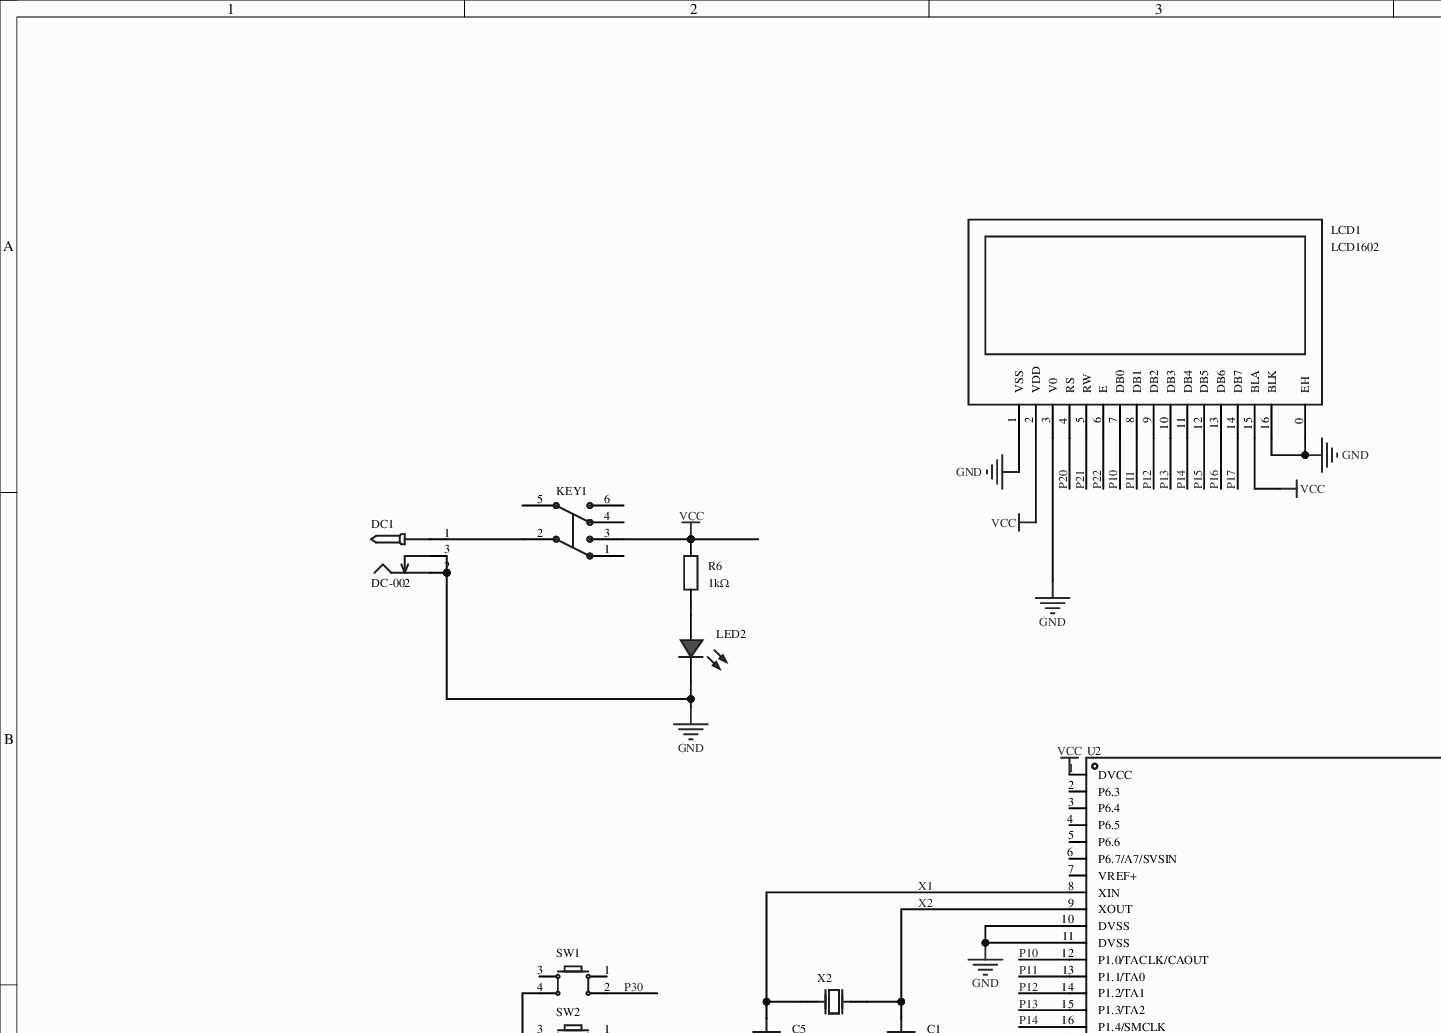
[diagram p0: MISC51174-3.schdoc, top left]
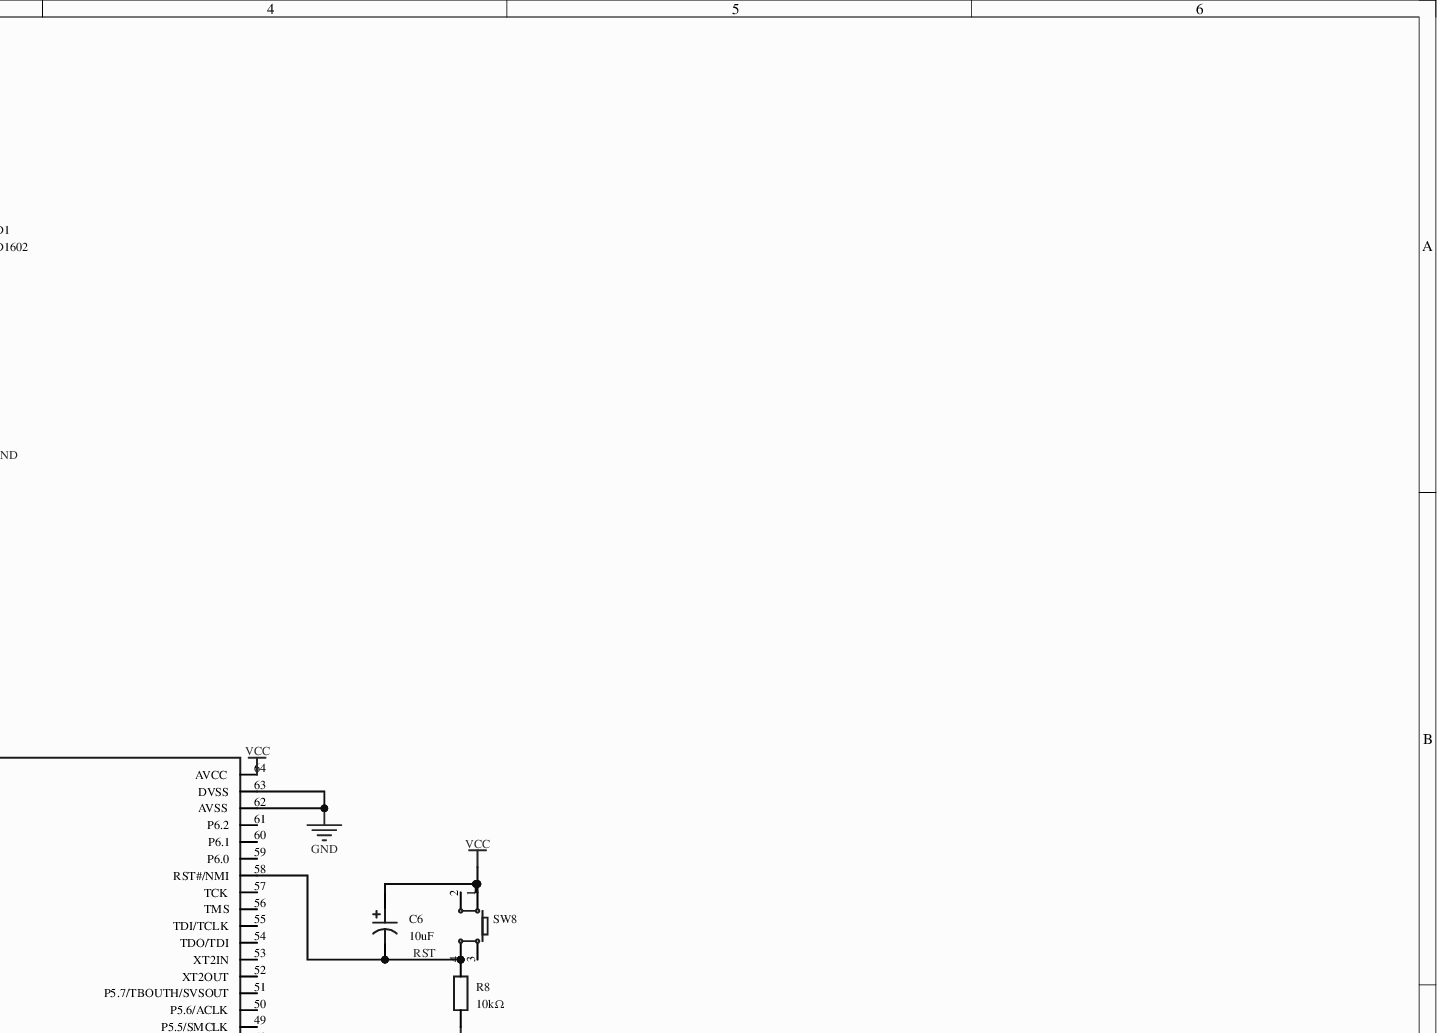
[diagram p1: MISC51174-3.schdoc, top right]
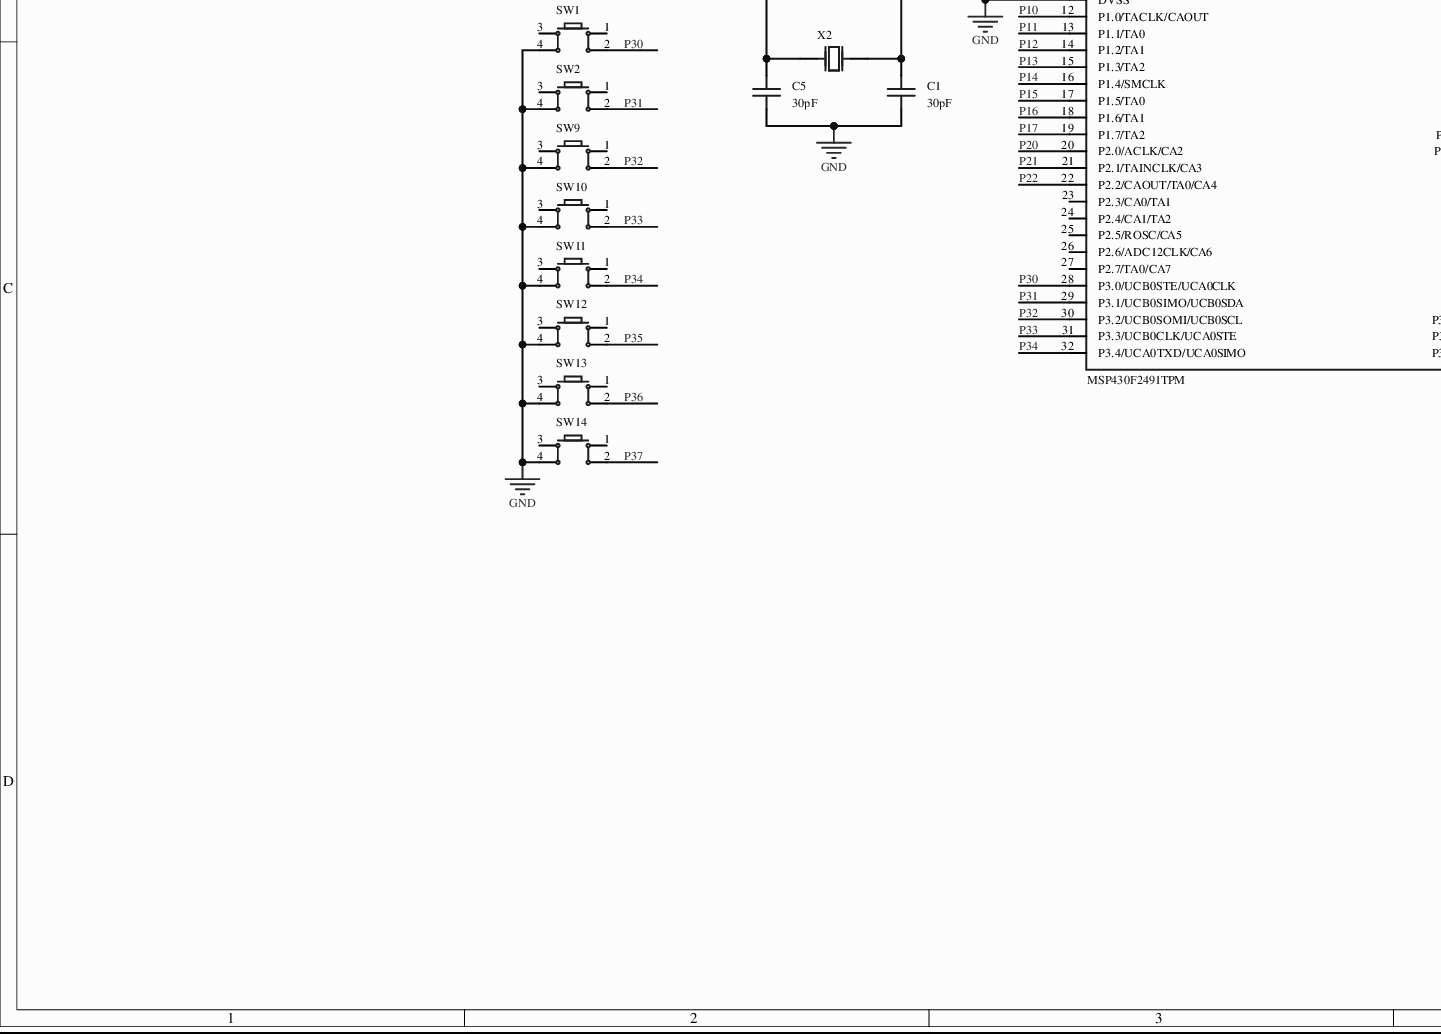
[diagram p2: MISC51174-3.schdoc, bottom left]
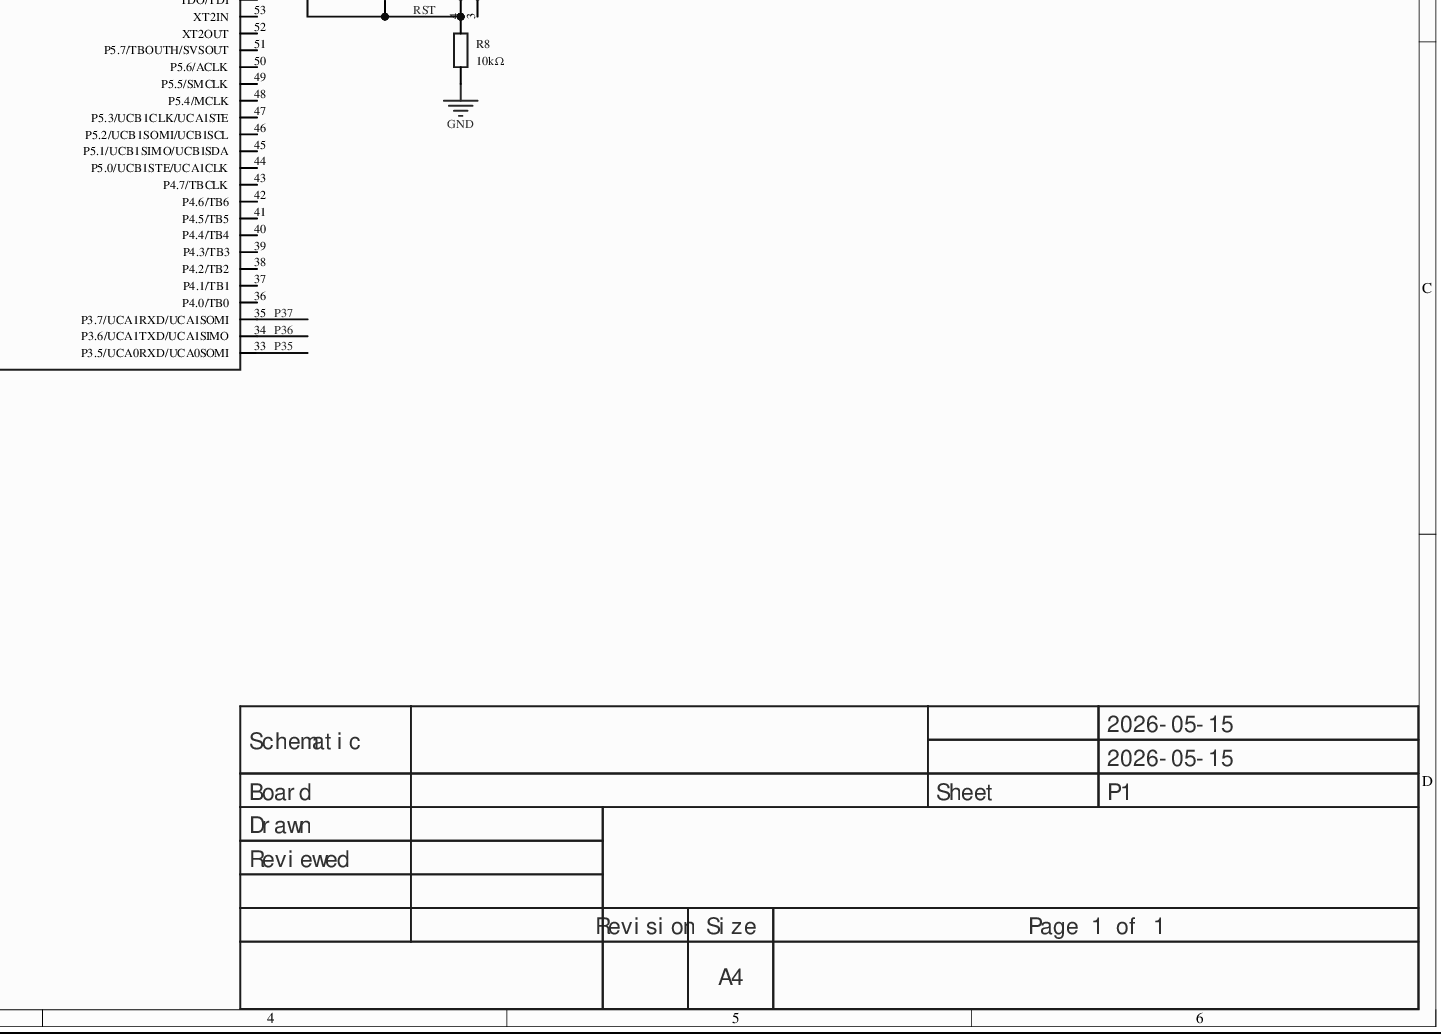
[diagram p3: MISC51174-3.schdoc, bottom right]
# Altium project MISC51174-2.PrjPcb
1 sheet, 20 parts. Net scope: global (net labels, ports and power ports of the same name join across sheets).
Board file: MISC51174.pcbdoc

## Sheet MISC51174-3.schdoc
size 420 x 297 mm; Version: V1.0; @Project Name: MISC51174; @Update Date: 2026-05-15; @Create Date: 2026-05-15; @Board Name: MISC51174; @Create Time: 10:13:01; @Page Count: 1; @Page No: 1; @Schematic Name: MISC51174; @Update Time: 10:13:01; Size: A4

### Parts
C1  30pF  [CAP-TH_L3.8-W2.5-P2.54-D0.50]
C5  30pF  [CAP-TH_L3.8-W2.5-P2.54-D0.50]
C6  10uF  [CAP-TH_BD5.0-P2.00-D0.8-FD-10UF50VC110GL]
DC1  DC-002  [DC-IN-TH_DC-3510]
KEY1  Non-latching switch 8.5×8.5 silent  [SW-TH_6P-L8.5-W8.5-P2.54]  (value not drawn)
LCD1  LCD1602  [LCD1602]
LED2  (no value)  [LED_TH-3mm]
R6  1kΩ  [Res_1/8W]
R8  10kΩ  [Res_1/8W]
SW1  (no value)  [SW-TH_4P-L6.0-W6.0-P4.50-LS6.5]
SW2  (no value)  [SW-TH_4P-L6.0-W6.0-P4.50-LS6.5]
SW8  (no value)  [SW-TH_4P-L6.0-W6.0-P4.50-LS6.5]
SW9  (no value)  [SW-TH_4P-L6.0-W6.0-P4.50-LS6.5]
SW10  (no value)  [SW-TH_4P-L6.0-W6.0-P4.50-LS6.5]
SW11  (no value)  [SW-TH_4P-L6.0-W6.0-P4.50-LS6.5]
SW12  (no value)  [SW-TH_4P-L6.0-W6.0-P4.50-LS6.5]
SW13  (no value)  [SW-TH_4P-L6.0-W6.0-P4.50-LS6.5]
SW14  (no value)  [SW-TH_4P-L6.0-W6.0-P4.50-LS6.5]
U2  MSP430F2491TPM  [LQFP-64_L10.0-W10.0-P0.50-LS12.0-TL]
X2  11.0592MHz  [OSC-TH_L11.1-W4.7-P4.88]  (value not drawn)

### Nets
GND: C1.1 C5.1 DC1.2 DC1.3 LCD1.0(EH) LCD1.1(VSS) LCD1.3(V0) LCD1.16(BLK) LED2.2(A) R8.1 SW1.4 SW2.4 SW9.4 SW10.4 SW11.4 SW12.4 SW13.4 SW14.4 U2.10(DVSS) U2.11(DVSS) U2.62(AVSS) U2.63(DVSS)
VCC: C6.1 KEY1.3 LCD1.2(VDD) LCD1.15(BLA) R6.2 SW8.1 U2.1(DVCC) U2.64(AVCC)
P10: LCD1.7(DB0) U2.12(P1.0/TACLK/CAOUT)
P11: LCD1.8(DB1) U2.13(P1.1/TA0)
P12: LCD1.9(DB2) U2.14(P1.2/TA1)
P13: LCD1.10(DB3) U2.15(P1.3/TA2)
P14: LCD1.11(DB4) U2.16(P1.4/SMCLK)
P15: LCD1.12(DB5) U2.17(P1.5/TA0)
P16: LCD1.13(DB6) U2.18(P1.6/TA1)
P17: LCD1.14(DB7) U2.19(P1.7/TA2)
P20: LCD1.4(RS) U2.20(P2.0/ACLK/CA2)
P21: LCD1.5(RW) U2.21(P2.1/TAINCLK/CA3)
P22: LCD1.6(E) U2.22(P2.2/CAOUT/TA0/CA4)
P30: SW1.2 U2.28(P3.0/UCB0STE/UCA0CLK)
P31: SW2.2 U2.29(P3.1/UCB0SIMO/UCB0SDA)
P32: SW9.2 U2.30(P3.2/UCB0SOMI/UCB0SCL)
P33: SW10.2 U2.31(P3.3/UCB0CLK/UCA0STE)
P34: SW11.2 U2.32(P3.4/UCA0TXD/UCA0SIMO)
P35: SW12.2 U2.33(P3.5/UCA0RXD/UCA0SOMI)
P36: SW13.2 U2.34(P3.6/UCA1TXD/UCA1SIMO)
P37: SW14.2 U2.35(P3.7/UCA1RXD/UCA1SOMI)
RST: C6.2 R8.2 SW8.4 U2.58(RST#/NMI)
X1: C5.2 U2.8(XIN) X2.1(OSC1)
X2: C1.2 U2.9(XOUT) X2.2(OSC2)
NetDC1_1: DC1.1 KEY1.2
NetLED2_1: LED2.1(C) R6.1

Not connected (* = marked no-connect by the designer): KEY1 1 4 5 6; SW1 1 3; SW2 1 3; SW8 2 3; SW9 1 3; SW10 1 3; SW11 1 3; SW12 1 3; SW13 1 3; SW14 1 3; U2 2(P6.3) 3(P6.4) 4(P6.5) 5(P6.6) 6(P6.7/A7/SVSIN) 7(VREF+) 23(P2.3/CA0/TA1) 24(P2.4/CA1/TA2) 25(P2.5/ROSC/CA5) 26(P2.6/ADC12CLK/CA6) 27(P2.7/TA0/CA7) 36(P4.0/TB0) 37(P4.1/TB1) 38(P4.2/TB2) 39(P4.3/TB3) 40(P4.4/TB4) 41(P4.5/TB5) 42(P4.6/TB6) 43(P4.7/TBCLK) 44(P5.0/UCB1STE/UCA1CLK) 45(P5.1/UCB1SIMO/UCB1SDA) 46(P5.2/UCB1SOMI/UCB1SCL) 47(P5.3/UCB1CLK/UCA1STE) 48(P5.4/MCLK) 49(P5.5/SMCLK) 50(P5.6/ACLK) 51(P5.7/TBOUTH/SVSOUT) 52(XT2OUT) 53(XT2IN) 54(TDO/TDI) 55(TDI/TCLK) 56(TMS) 57(TCK) 59(P6.0) 60(P6.1) 61(P6.2)

### Notes on the sheet
- 2026-05-15
- Schematic
- Board
- Sheet
- P1
- Drawn
- Reviewed
- Revision
- Size
- A4
- Page 1 of 1

### Library data of the parts
C1 C5 = C315C300K3G5TA7301: Capacitance:30pF;Tolerance:±10%;Rated voltage:25V;Temperature coefficient:C0G;; Manufacturer: KEMET(基美); 3D Model: 0be8c650c9044d099e9add656cc6dda60819f05c4eef4c71ace90d822a990e87; 3D Model Transform: 149.606,98.8187,0,0,0,0,0,0,-196.85; Tolerance: ±10%; Voltage Rating: 25V; Temperature Coefficient: C0G; Pin Spacing: 2.54mm; AddInBom: yes; Symbol: C315C300K3G5TA7301; Device: C315C300K3G5TA7301; LCSC Part Name: 30pF ±10% 25V; Supplier Part: C2245291; Manufacturer Part: C315C300K3G5TA7301; Supplier Footprint: 插件,P=2.54mm; JLCPCB Part Class: Extended Part; Datasheet: https://item.szlcsc.com/datasheet/C315C300K3G5TA7301/2337370.html; Supplier: LCSC; Value: 30pF; ConvertToPcb: yes; FootprintName: CAP-TH_L3.8-W2.5-P2.54-D0.50; ModelName: CAP-TH_L3.8-W2.5-P2.54-D0.50
C6 = 10UF50VC110GL: Capacitance:10uF;Tolerance:±20%;Rated voltage:50V;Ripple current:120mA@100KHz;Equivalent series resistance (ESR):1.6Ω;; Manufacturer: Econd(米朗电子); Tolerance: ±20%; Voltage Rating: 50V; Equivalent Series Resistance(ESR): 1.6Ω; Pin Spacing: 2mm; Lifetime: 5000hrs@105℃; AddInBom: yes; Symbol: 10UF50VC110GL; Device: 10UF50VC110GL; LCSC Part Name: 10uF ±20% 50V; Supplier Part: C46867109; Manufacturer Part: 10UF50VC110GL; Supplier Footprint: 插件,D5xL11mm; JLCPCB Part Class: Extended Part; Datasheet: https://item.szlcsc.com/datasheet/10UF50VC110GL/49031974.html; Supplier: LCSC; Value: 10uF; Ripple Current: 120mA@100KHz; Diameter: 5mm; Height - Seated (Max): 11mm; Operating Temperature: -40℃~+105℃; ConvertToPcb: yes; FootprintName: CAP-TH_BD5.0-P2.00-D0.8-FD-10UF50VC110GL
DC1 = DC-002: 3D Model: 28059cb5f325411c86e5e1af88d5b1310819f05c4eef4c71ace90d822a990e87; 3D Model Transform: 450.787,208.661,0,180,0,0,113.189,-47.244,-125.984; AddInBom: yes; Symbol: DC-002; Device: DC-002; LCSC Part Name: DC-002 铁脚 内铁芯1.0mm; Supplier Part: C12568; Manufacturer Part: DC-002; Supplier Footprint: 插件; JLCPCB Part Class: Extended Part; Supplier: LCSC; ConvertToPcb: yes; FootprintName: DC-IN-TH_DC-3510; ModelName: DC-IN-TH_DC-3510
KEY1 = 无自锁开关 8.5×8.5 无声: 6 pins, 8.5×8.5; Symbol: No self-locking switch 8.5×8.5 silent; 3D Model: 4c72b3966b92446eb355e1bd0fb4f8800819f05c4eef4c71ace90d822a990e87; 3D Model Transform: 342.519,334.645,0,180,0,0,0,0,-137.795; AddInBom: yes; Device: Non-latching switch 8.5×8.5 silent; LCSC Part Name: 无自锁开关 8.5×8.5  无声; Supplier Part: C26228; Manufacturer Part: 无自锁开关 8.5×8.5 无声; Supplier Footprint: 插件; JLCPCB Part Class: Extended Part; Supplier: LCSC; ConvertToPcb: yes; FootprintName: SW-TH_6P-L8.5-W8.5-P2.54; ModelName: SW-TH_6P-L8.5-W8.5-P2.54
LCD1 = HS1602A: Controller:SPLC780;Size(inch):2;; Manufacturer: HS(汉昇); 3D Model: f9d832f46a914cadb50fc4d4cefd25170819f05c4eef4c71ace90d822a990e87; 3D Model Transform: 3149.6,1417.32,0,0,0,0,0,0,-118.11; AddInBom: yes; Symbol: HS1602A; Device: HS1602A; LCSC Part Name: 2.0寸16*2单色字符字符液晶显示屏; Supplier Part: C5329588; Manufacturer Part: LCD1602; Supplier Footprint: -; JLCPCB Part Class: Extended Part; Datasheet: https://atta.szlcsc.com/upload/public/pdf/source/20221212/35734F14DBB323F90DD8DBE1717CD9FD.pdf; Supplier: LCSC; Main Control Chip: SPLC780; Size: 2; Operating Temperature: -20℃~+70℃; ConvertToPcb: yes; FootprintName: LCD1602; ModelName: LCD1602
LED2 = LED_TH-R_3mm: 3D Model: a497c992633541038a38947cdc58012f0819f05c4eef4c71ace90d822a990e87; 3D Model Transform: 141.274,153.327,0,0,0,0,-5.984,0,-137.795; ConvertToPcb: yes; ModelName: LED-TH-3mm_R; Symbol: LED_TH-R; Device: LED_TH-R_3mm; Supplier Footprint: 插件; AddInBom: yes; FootprintName: LED_TH-3mm
R6 R8 = Res_AXIAL-1/8W: Symbol: Resistor; 3D Model: b2b5ae7ae4c642178fe0039925c86a3f0819f05c4eef4c71ace90d822a990e87; 3D Model Transform: 282.86,66.88,253.09,0,0,0,0,0,-191; ConvertToPcb: yes; ModelName: RES-TH_BD1.8-L3.2-P7.20-D0.4; Device: Res_AXIAL-1/8W; Supplier Footprint: 轴向引线; AddInBom: yes; FootprintName: Res_1/8W
  R6: Value: 1kΩ
  R8: Value: 10kΩ
SW1 SW2 SW8-SW14 = Key_TH_6x6x6: Contact current:50mA;Rated voltage (DC):12V;Insulation resistance:100MΩ;Circuit structure:SPST;Mounting:Through-hole;Button shape:Round button;Button/cap colour:Black;Actuation force:260gf@±30gf;Operating temperature:-25℃~+70℃;Pin style:PC pin;Switch length:6mm;Switch width:6mm;Switch height:6mm;With bracket:No;; Symbol: Tactile switch; 3D Model: 20eee248bc684ccd8cbdbb1d0d91ec6f0819f05c4eef4c71ace90d822a990e87; 3D Model Transform: 236.22,323.03,0,90,0,0,0,0,-137.795; AddInBom: yes; ModelName: SW-TH_4P-L6.0-W6.0-H5.0-LS6.5-P4.50; Device: Key_TH_6x6x6; Supplier Footprint: 插件; ConvertToPcb: yes; FootprintName: SW-TH_4P-L6.0-W6.0-P4.50-LS6.5
U2 = MSP430F2491TPM: CPU core:MSP430;Program memory:60KB;Total RAM:2KB;GPIO ports:48;Operating voltage:1.8V~3.6V;CPU max frequency:16MHz;Program memory type:-;; Manufacturer: TI(德州仪器); AddInBom: yes; ModelId: cd9de06618c44fcf82654c43a457f83c0819f05c4eef4c71ace90d822a990e87; ModelName: LQFP-64_L10.0-W10.0-H1.4-LS12.0-P0.50; ModelTransform: 472.441,472.441,0,270,0,0,0,0,0; CPU Core: MSP430; Program Storage Size: 60KB; RAM Size: 2KB; GPIO Ports Number: 48; CPU Maximum Speed: 16MHz; Peripheral/Function: Watchdog; LIN bus protocol; PWM; IrDA; Symbol: MSP430F2491TPM; Device: MSP430F2491TPM; LCSC Part Name: 具有 60KB 闪存、2KB SRAM、比较器、I2C/SPI/UART 和硬件乘法器的 16MHz MCU; SupplierPart: C1344424; ManufacturerPart: MSP430F2491TPM; Supplier Footprint: LQFP-64(10x10); JLCPCB Part Class: Extended Part; Supplier: LCSC; ConvertToPcb: yes; FootprintName: LQFP-64_L10.0-W10.0-P0.50-LS12.0-TL; Operating Voltage Range: 1.8V~3.6V; Program Memory Type: -; Operating Temperature Range: -40℃~+105℃; ADC (Bit): -; DAC (Bit): -; PWM (Bit): -; 8Bit Timer: -; 16Bit Timer: -; 32Bit Timer: -; CAN: -; UART/USART: -; I2C: -; I2S: -; SPI: -; Universal Serial Bus: -; Internal Comparator: -; communication protocol: -; Watchdog: Yes; Real-Time Clock: -; Infrared Data Association: Yes; Low-Voltage Detect: Yes; CCP Capture/Compare: -; Secure Digital Input and Output: -; Direct Memory Access: -; Internal Oscillator: Yes
X2 = 9AC11059302060C3: Crystal type:Through-hole crystal;Frequency:11.0592MHz;Frequency tolerance (room temp):±20ppm;Load capacitance:30pF;; Manufacturer: JGHC(晶光华); 3D Model: f2ed30de83344a4b83b1c4b1b9fe18560819f05c4eef4c71ace90d822a990e87; 3D Model Transform: 436.37503,185.039,0,0,0,0,0,0,-137.795; Normal temperature Frequency Tolerance: ±20ppm; Load Capacitance: 30pF; Equivalent Series Resistance(ESR): 60Ω; AddInBom: yes; Symbol: 9AC11059302060C3; Device: 9AC11059302060C3; LCSC Part Name: 11.0592MHz ±20ppm 30pF; Supplier Part: C2715911; Manufacturer Part: 9AC11059302060C3; Supplier Footprint: HC-49S; JLCPCB Part Class: Extended Part; Datasheet: https://item.szlcsc.com/datasheet/9AC11059302060C3/2832137.html; Supplier: LCSC; Type: Through-hole crystal; Value: 11.0592MHz; Operating Temperature: -40℃~+85℃; ConvertToPcb: yes; FootprintName: OSC-TH_L11.1-W4.7-P4.88; ModelName: OSC-TH_L11.1-W4.7-P4.88